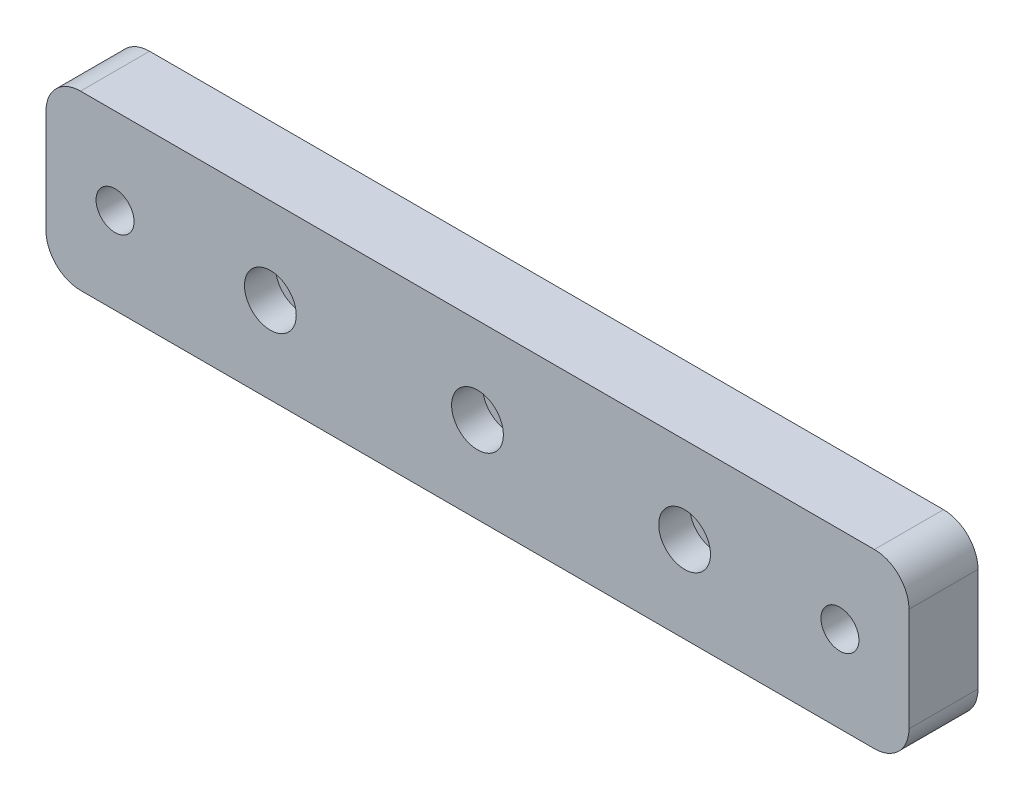
SolidWorks part; units mm, degrees
ref_plane "Front Plane" through (0, 0, 0) normal (0, 0, 1) x (1, 0, 0)
ref_plane "Top Plane" through (0, 0, 0) normal (0, 1, 0) x (1, 0, 0)
ref_plane "Right Plane" through (0, 0, 0) normal (1, 0, 0) x (0, 0, -1)
other "Configuration Table"
sketch "Sketch1" plane through (0, 0, 0) normal (0, 0, 1) x (1, 0, 0)
  line L1 (75, -25) -> (-175, -25)
  line L2 (75, -25) -> (75, 25)
  line L3 (75, 25) -> (-175, 25)
  line L4 (-175, -25) -> (-175, 25)
  line L5 (75, -25) -> (-175, 25) construction
  line L6 (75, 25) -> (-175, -25) construction
  point P0 (-50, 0)
  dimension "D1" = 50
  dimension "D2" = 250
extrude "Boss-Extrude1" add sketch "Sketch1" along normal blind 20
fillet "Fillet1" radius 10 4 edges at (75, -25, 10) (-175, -25, 10) (-175, 25, 10) (75, 25, 10)
hole_wizard "CBORE for M8 Hexagon socket head cap screws1" positions "3DSketch1" profile "Sketch2" counterbore size "M8" standard "GB"
sketch3d "3DSketch1"
  line L0 (-50, 25, 20) -> (-50, -25, 20) construction
  line L1 (65, 25, 20) -> (-165, 25, 20) construction
  line L3 (-165, -25, 20) -> (65, -25, 20) construction
  point P0 (10, 0, 20)
  point P19 (-50, 0, 20)
  dimension "D1" = 60
sketch "Sketch2" plane through (10, 0, 20) normal (1, 0, 0) x (0, -1, 0)
  line L0 (0, 0) -> (0, 24.9539)
  line L1 (0, 24.9539) -> (4.5, 22.25)
  line L2 (4.5, 22.25) -> (4.5, 9)
  line L3 (4.5, 9) -> (7.5, 9)
  line L4 (7.5, 9) -> (7.5, 0)
  line L5 (7.5, 0) -> (0, 0)
  line L10 (0, 24.9539) -> (-4.5, 22.25) construction
  line L11 (0, -6.35) -> (0, 107.95) construction
  dimension "孔直径" = 9
  dimension "孔深度" = 22.25
  dimension "柱形沉头孔直径" = 15
  dimension "柱形沉头孔深度" = 9
  dimension "导头角度" = 118
pattern_linear "LPattern1" count 3 spacing 60 along (-1, 0, 0) of "CBORE for M8 Hexagon socket head cap screws1"
hole_wizard "CBORE for M10 Hexagon socket head cap screws1" positions "3DSketch2" profile "Sketch4" counterbore size "M10" standard "GB"
sketch3d "3DSketch2"
  line L0 (75, -15, 0) -> (75, 15, 0) construction
  line L1 (-175, 15, 0) -> (-175, -15, 0) construction
  point P0 (55, 0, 0)
  point P2 (-155, 0, 0)
  point P10 (75, 0, 0)
  dimension "D1" = 20
  dimension "D2" = 20
sketch "Sketch4" plane through (55, 0, 0) normal (1, 0, 0) x (0, 1, 0)
  line L0 (0, 0) -> (0, 30.8047)
  line L1 (0, 30.8047) -> (5.5, 27.5)
  line L2 (5.5, 27.5) -> (5.5, 11)
  line L3 (5.5, 11) -> (9, 11)
  line L5 (9, 11) -> (9, 0.025)
  line L6 (9, 0.025) -> (9.025, 0)
  line L7 (9.025, 0) -> (0, 0)
  line L8 (-9, 0.025) -> (-9.025, 0) construction
  line L10 (0, 30.8047) -> (-5.5, 27.5) construction
  line L11 (0, -6.35) -> (0, 107.95) construction
  dimension "孔直径" = 11
  dimension "孔深度" = 27.5
  dimension "锥形沉头孔直径" = 18
  dimension "锥形沉头孔深度" = 11
  dimension "近端锥形沉头孔直径" = 18.05
  dimension "近端锥形沉头孔角度" = 90
  dimension "导头角度" = 118
